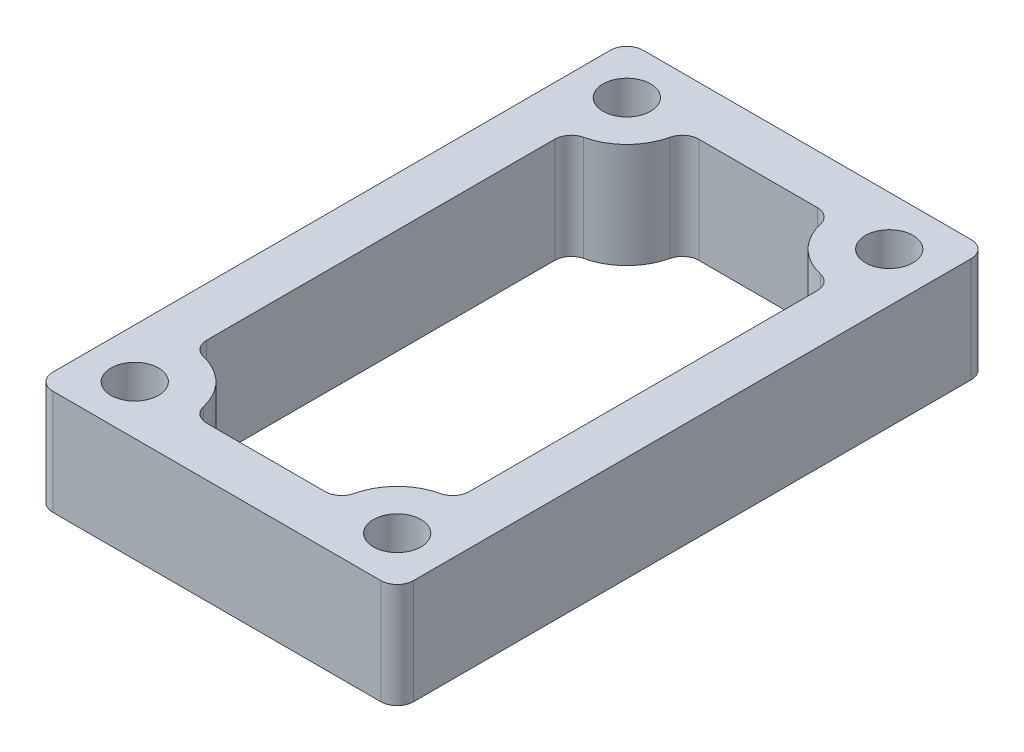
from build123d import *

# Parameters (mm, degrees)
SKETCH_1_W      = 22
SKETCH_1_H      = 36
SKETCH_1_R      = 1.45
EXTRUDE_1_DEPTH = 6.4
FILLET_1_R      = 1
FILLET_2_R      = 1


with BuildPart() as part:
    # 草图1 → 凸台-拉伸1 (new body)
    with BuildSketch(Plane(origin=(0, 0, 0), x_dir=(1, 0, 0), z_dir=(0, 1, 0))):
        Rectangle(SKETCH_1_W, SKETCH_1_H)
        with Locations(Location((-8, 15, 0), (0, 0, 270))):
            Circle(SKETCH_1_R, mode=Mode.SUBTRACT)
        with Locations(Location((8, 15, 0), (0, 0, 270))):
            Circle(SKETCH_1_R, mode=Mode.SUBTRACT)
        with Locations(Location((-8, -15, 0), (0, 0, 270))):
            Circle(SKETCH_1_R, mode=Mode.SUBTRACT)
        with Locations(Location((8, -15, 0), (0, 0, 270))):
            Circle(SKETCH_1_R, mode=Mode.SUBTRACT)
        with BuildLine():
            Line((-4.5, 15), (4.5, 15))
            ThreePointArc((4.5, 15), (5.525126266, 12.525126266), (8, 11.5))
            Line((8, 11.5), (8, -11.5))
            ThreePointArc((8, -11.5), (5.525126266, -12.525126266), (4.5, -15))
            Line((4.5, -15), (-4.5, -15))
            ThreePointArc((-4.5, -15), (-5.525126266, -12.525126266), (-8, -11.5))
            Line((-8, -11.5), (-8, 11.5))
            ThreePointArc((-8, 11.5), (-5.525126266, 12.525126266), (-4.5, 15))
        make_face(mode=Mode.SUBTRACT)
    extrude(amount=EXTRUDE_1_DEPTH)

    # 圆角1
    fillet_1_edges = [part.edges().sort_by_distance(p)[0] for p in [
        (8, 3.2, -11.5),
        (4.5, 3.2, -15),
        (-4.5, 3.2, -15),
        (-8, 3.2, -11.5),
        (-8, 3.2, 11.5),
        (-4.5, 3.2, 15),
        (4.5, 3.2, 15),
        (8, 3.2, 11.5),
    ]]
    fillet(fillet_1_edges, radius=FILLET_1_R)

    # 圆角2
    fillet_2_edges = [part.edges().sort_by_distance(p)[0] for p in [
        (-11, 3.2, -18),
        (11, 3.2, -18),
        (11, 3.2, 18),
        (-11, 3.2, 18),
    ]]
    fillet(fillet_2_edges, radius=FILLET_2_R)


solid = part.part
